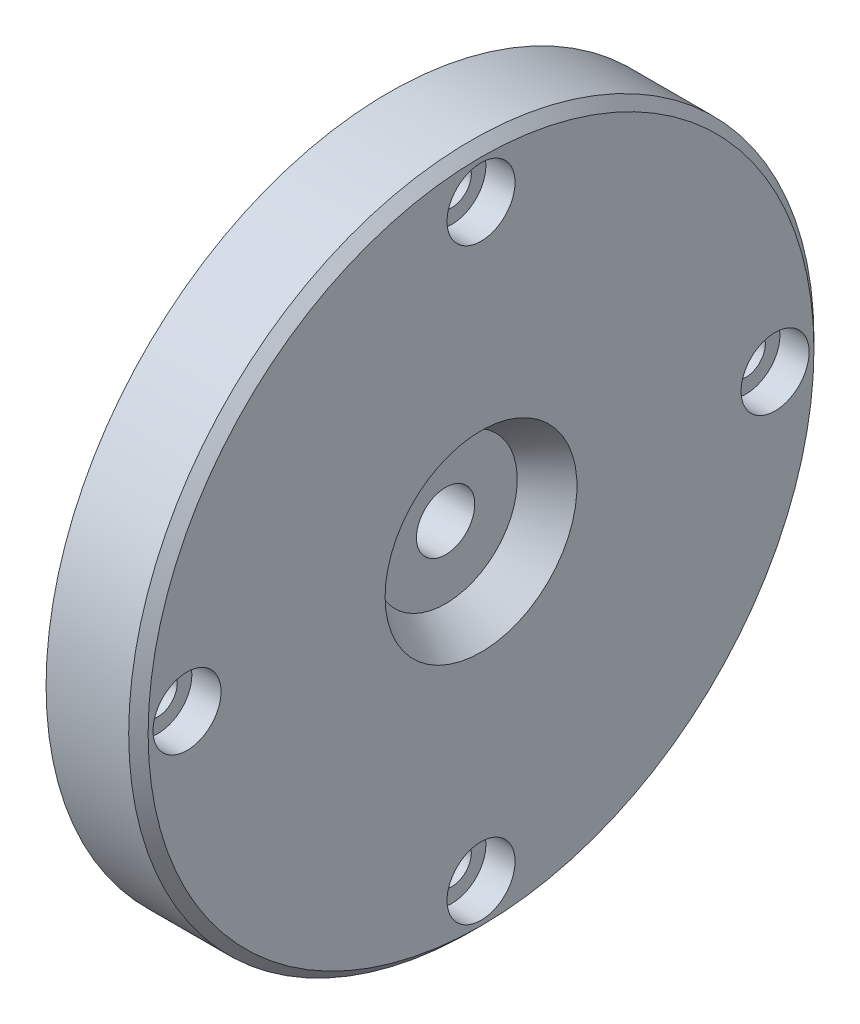
SolidWorks part; units mm, degrees
ref_plane "Front Plane" through (0, 0, 0) normal (0, 0, 1) x (1, 0, 0)
ref_plane "Top Plane" through (0, 0, 0) normal (0, 1, 0) x (1, 0, 0)
ref_plane "Right Plane" through (0, 0, 0) normal (1, 0, 0) x (0, 0, -1)
sketch "Sketch1" plane through (0, 0, 0) normal (0, 0, 1) x (1, 0, 0)
  line L0 (-75.3944, 0) -> (92.8892, 0) construction
  line L1 (-28.7415, 6) -> (-28.7415, 51.5)
  line L2 (-28.7415, 51.5) -> (-21.7415, 51.5)
  line L3 (-21.7415, 51.5) -> (-21.7415, 70.5)
  line L4 (-21.7415, 70.5) -> (-2.7415, 70.5)
  line L5 (-2.7415, 70.5) -> (-2.7415, 19.7459)
  line L6 (-2.7415, 19.7459) -> (-10.031, 14.7474)
  line L7 (-10.031, 14.7474) -> (-10.031, 6)
  line L8 (-10.031, 6) -> (-28.7415, 6)
  dimension "D1" = 70.5
  dimension "D2" = 51.5
  dimension "D3" = 6
  dimension "D4" = 26
  dimension "D5" = 19
revolve "Revolve1" add sketch "Sketch1" angle 360 about L0
chamfer "Chamfer1" distance 2 angle 45 1 edges at (-2.7415, 0, 70.5)
sketch "Sketch2" plane through (-2.7415, 0, 0) normal (1, 0, 0) x (0, 0, -1)
  circle A1 centre (0, -60.5) radius 4
  circle A2 centre (-60.5, 0) radius 4
  circle A3 centre (0, 60.5) radius 4
  circle A4 centre (60.5, 0) radius 4
  point P14 (0, 0)
  dimension "D2" = 8
  dimension "D3" = 4
extrude "Cut-Extrude1" cut sketch "Sketch2" against normal blind 49
sketch "Sketch3" plane through (-2.7415, 0, 0) normal (1, 0, 0) x (0, 0, -1)
  circle A0 centre (-60.5, 0) radius 7
  circle A1 centre (0, 60.5) radius 7
  circle A2 centre (60.5, 0) radius 7
  circle A3 centre (0, -60.5) radius 7
  dimension "D1" = 14
  dimension "D2" = 14
  dimension "D3" = 14
  dimension "D4" = 14
extrude "Cut-Extrude2" cut sketch "Sketch3" against normal blind 6
